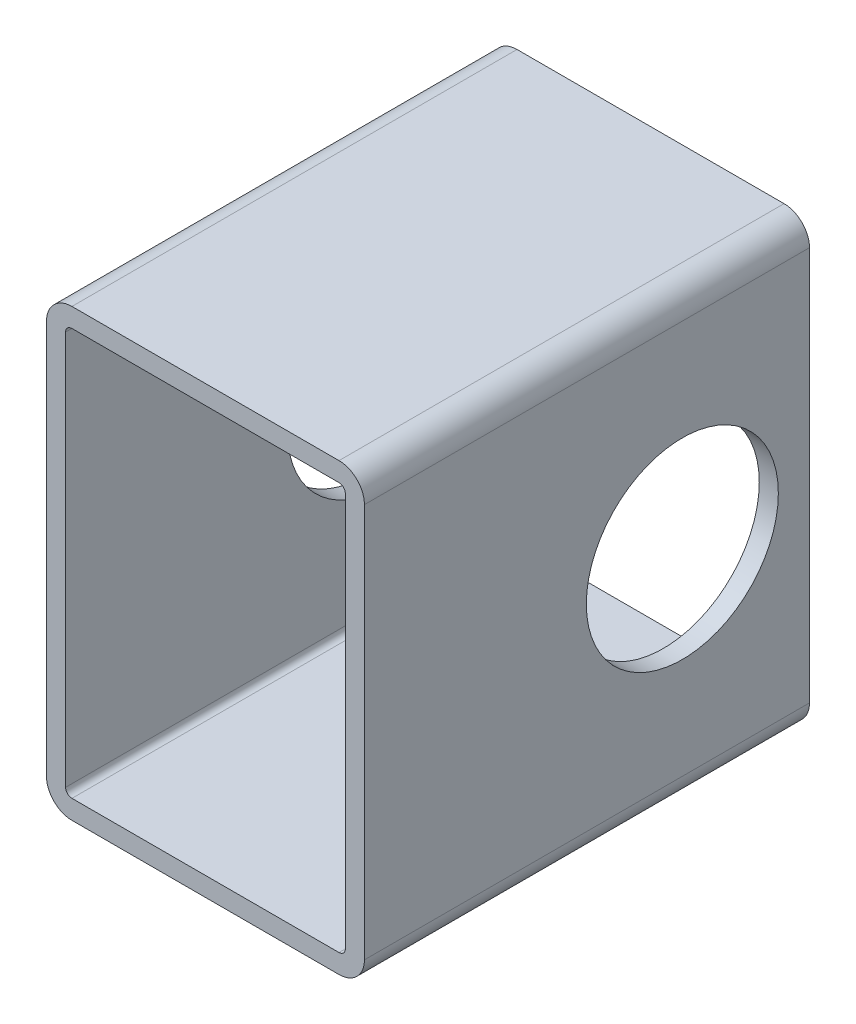
SolidWorks part; units mm, degrees
material "AISI 1045 钢，冷拔"
ref_plane "Front Plane" through (0, 0, 0) normal (0, 0, 1) x (1, 0, 0)
ref_plane "Top Plane" through (0, 0, 0) normal (0, 1, 0) x (1, 0, 0)
ref_plane "Right Plane" through (0, 0, 0) normal (1, 0, 0) x (0, 0, -1)
sketch "Sketch1" plane through (0, 0, 0) normal (0, 0, 1) x (1, 0, 0)
  line L1 (-21, -35) -> (21, -35)
  line L2 (-25, -31) -> (-25, 31)
  line L3 (-21, 35) -> (21, 35)
  line L4 (25, -31) -> (25, 31)
  line L5 (-25, -35) -> (25, 35) construction
  line L6 (-25, 35) -> (25, -35) construction
  arc A0 (-21, -35) -> (-25, -31) centre (-21, -31) cw
  arc A1 (21, -35) -> (25, -31) centre (21, -31) ccw
  arc A2 (21, 35) -> (25, 31) centre (21, 31) cw
  arc A3 (-25, 31) -> (-21, 35) centre (-21, 31) cw
  point P0 (0, 0)
  dimension "D3" = 4
  dimension "D1" = 50
  dimension "D2" = 70
extrude "Extrude-Thin1" add sketch "Sketch1" along normal blind 70 thin thin type one direction reverse wall 3
sketch "Sketch2" plane through (25, 0, 0) normal (1, 0, 0) x (0, 0, -1)
  line L0 (0, -31) -> (0, 31) construction
  line L1 (-70, 35) -> (0, 35) construction
  circle A0 centre (-20, 0) radius 15.1
  dimension "D1" = 30.2
  dimension "D2" = 20
  dimension "D3" = 35
extrude "Cut-Extrude1" cut sketch "Sketch2" against normal through all
